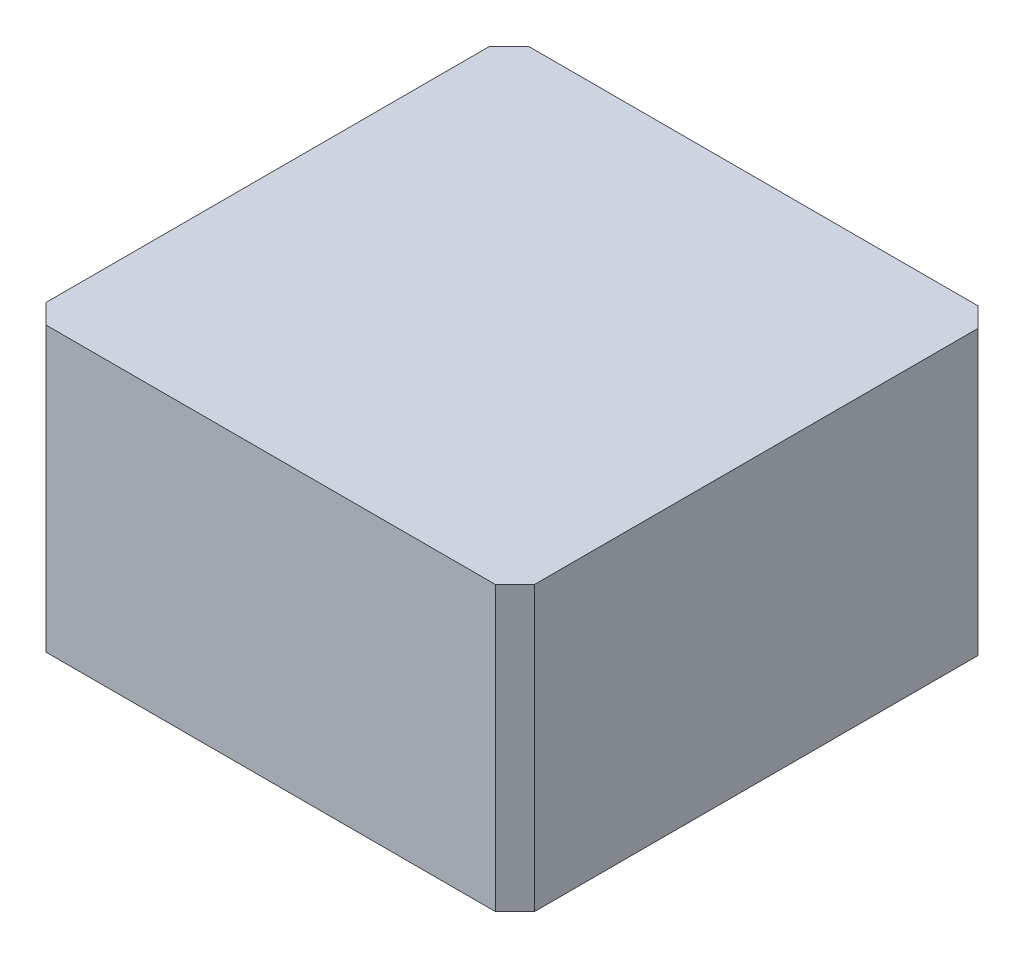
from build123d import *

# Parameters (mm, degrees)
SKETCH1_W           = 250
SKETCH1_H           = 247
BOSS_EXTRUDE1_DEPTH = 145
CHAMFER1_SIZE       = 10
SKETCH3_W           = 212
SKETCH3_H           = 210
SKETCH3_W_2         = 202
SKETCH3_H_2         = 200
CUT_EXTRUDE2_DEPTH  = 1


with BuildPart() as part:
    # Sketch1 → Boss-Extrude1 (new body)
    with BuildSketch(Plane(origin=(0, 0, 0), x_dir=(1, 0, 0), z_dir=(0, 1, 0))):
        Rectangle(SKETCH1_W, SKETCH1_H)
    extrude(amount=BOSS_EXTRUDE1_DEPTH)

    # Chamfer1
    chamfer1_edges = [part.edges().sort_by_distance(p)[0] for p in [
        (125, 72.5, 123.5),
        (-125, 72.5, 123.5),
        (-125, 72.5, -123.5),
        (125, 72.5, -123.5),
    ]]
    chamfer(chamfer1_edges, length=CHAMFER1_SIZE)

    # Sketch3 → Cut-Extrude2 (cut)
    with BuildSketch(Plane.XZ):
        Rectangle(SKETCH3_W, SKETCH3_H)
        Rectangle(SKETCH3_W_2, SKETCH3_H_2, mode=Mode.SUBTRACT)
    extrude(amount=-CUT_EXTRUDE2_DEPTH, mode=Mode.SUBTRACT)


solid = part.part
